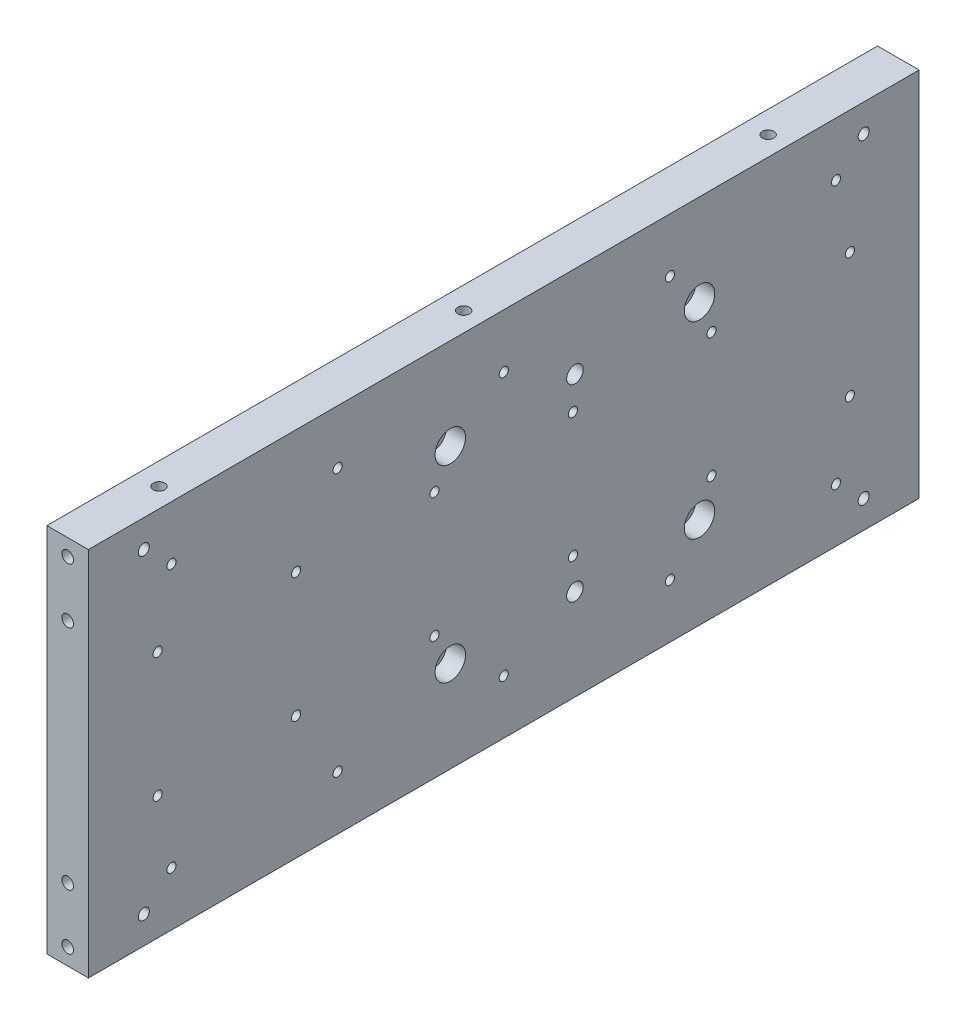
from build123d import *

# Parameters (mm, degrees)
SKETCH1_W                                            = 300
SKETCH1_H                                            = 134
BOSS_EXTRUDE1_DEPTH                                  = 15
M4_TAPPED_HOLE1_D                                    = 3.3
M4_TAPPED_HOLE1_DEPTH                                = 10.1
M4_TAPPED_HOLE1_TIP                                  = 0.991420021
M4_TAPPED_HOLE2_D                                    = 3.3
M4_TAPPED_HOLE2_DEPTH                                = 10.1
M4_TAPPED_HOLE2_TIP                                  = 0.991420021
M5_TAPPED_HOLE1_AT_2_COUNT                           = 2
M5_TAPPED_HOLE1_AT_2_PITCH                           = 20
M5_TAPPED_HOLE1_AT_3_COUNT                           = 2
M5_TAPPED_HOLE1_AT_3_PITCH                           = 102
M5_TAPPED_HOLE1_AT_4_COUNT                           = 2
M5_TAPPED_HOLE1_AT_4_PITCH                           = 122
F_4_0MM_DOWEL_HOLE1_D                                = 4
F_4_0MM_DOWEL_HOLE1_DEPTH                            = 6
F_4_0MM_DOWEL_HOLE1_TIP                              = 1.201721238
CBORE_FOR_M6_HEXAGON_SOCKET_HEAD_CAP_SCR_D           = 6.6
CBORE_FOR_M6_HEXAGON_SOCKET_HEAD_CAP_SCR_CBORE_D     = 11
CBORE_FOR_M6_HEXAGON_SOCKET_HEAD_CAP_SCR_CBORE_DEPTH = 6.8
F_6_0MM_DOWEL_HOLE1_D                                = 6
M5_TAPPED_HOLE2_D                                    = 4.2
M5_TAPPED_HOLE2_DEPTH                                = 12.4
M5_TAPPED_HOLE2_TIP                                  = 1.2618073


with BuildPart() as part:
    # Sketch1 → Boss-Extrude1 (new body)
    with BuildSketch(Plane(origin=(0, 0, 0), x_dir=(0, 0, -1), z_dir=(1, 0, 0))):
        Rectangle(SKETCH1_W, SKETCH1_H)
    extrude(amount=BOSS_EXTRUDE1_DEPTH)

    # M4 Tapped Hole1
    with Locations(Plane(origin=(15, 0, 0), x_dir=(0, 0, -1), z_dir=(1, 0, 0))):
        with Locations((-120, -47.5), (-60, -47.5), (0, -47.5), (60, -47.5), (120, -47.5), (120, 47.5), (60, 47.5), (0, 47.5), (-60, 47.5), (-120, 47.5)):
            Hole(M4_TAPPED_HOLE1_D / 2, depth=M4_TAPPED_HOLE1_DEPTH)
            with Locations((0, 0, -(M4_TAPPED_HOLE1_DEPTH + M4_TAPPED_HOLE1_TIP / 2))):  # 118° drill point
                Cone(0, M4_TAPPED_HOLE1_D / 2, M4_TAPPED_HOLE1_TIP, mode=Mode.SUBTRACT)

    # M4 Tapped Hole2
    with Locations(Plane(origin=(15, 0, 0), x_dir=(0, 0, -1), z_dir=(1, 0, 0))):
        with Locations((-125, 22.5), (-75, 22.5), (-25, 22.5), (-125, -22.5), (-75, -22.5), (-25, -22.5), (25, 22.5), (75, 22.5), (125, 22.5), (125, -22.5), (75, -22.5), (25, -22.5)):
            Hole(M4_TAPPED_HOLE2_D / 2, depth=M4_TAPPED_HOLE2_DEPTH)
            with Locations((0, 0, -(M4_TAPPED_HOLE2_DEPTH + M4_TAPPED_HOLE2_TIP / 2))):  # 118° drill point
                Cone(0, M4_TAPPED_HOLE2_D / 2, M4_TAPPED_HOLE2_TIP, mode=Mode.SUBTRACT)

    # Sketch7 → M5 Tapped Hole1 (revolve, cut)
    with BuildSketch(Plane(origin=(7.5, -61, -150), x_dir=(0, 1, 0), z_dir=(1, 0, 0))):
        Polygon((0, 0), (0, 13.6618073), (2.1, 12.4), (2.1, 0), align=None)
    m5_tapped_hole1 = revolve(axis=Axis((7.5, -61, -156.35), (0, 0, 1)), mode=Mode.SUBTRACT)

    # M5 Tapped Hole1 at 2: M5 Tapped Hole1 ×2
    with Locations(*[(0, i * M5_TAPPED_HOLE1_AT_2_PITCH, 0) for i in range(1, M5_TAPPED_HOLE1_AT_2_COUNT)]):
        add(m5_tapped_hole1, mode=Mode.SUBTRACT)

    # M5 Tapped Hole1 at 3: M5 Tapped Hole1 ×2
    with Locations(*[(0, i * M5_TAPPED_HOLE1_AT_3_PITCH, 0) for i in range(1, M5_TAPPED_HOLE1_AT_3_COUNT)]):
        add(m5_tapped_hole1, mode=Mode.SUBTRACT)

    # M5 Tapped Hole1 at 4: M5 Tapped Hole1 ×2
    with Locations(*[(0, i * M5_TAPPED_HOLE1_AT_4_PITCH, 0) for i in range(1, M5_TAPPED_HOLE1_AT_4_COUNT)]):
        add(m5_tapped_hole1, mode=Mode.SUBTRACT)

    # Mirror1: M5 Tapped Hole1 across plane
    add(m5_tapped_hole1.mirror(Plane.XY), mode=Mode.SUBTRACT)

    # Mirror1 copy 1 sketch → Mirror1 copy 1 (revolve, cut)
    with BuildSketch(Plane(origin=(7.5, -41, 150), x_dir=(0, 1, 0), z_dir=(1, 0, 0))):
        Polygon((0, 0), (0, -13.6618073), (2.1, -12.4), (2.1, 0), align=None)
    revolve(axis=Axis((7.5, -41, 156.35), (0, 0, 1)), mode=Mode.SUBTRACT)

    # Mirror1 copy 2 sketch → Mirror1 copy 2 (revolve, cut)
    with BuildSketch(Plane(origin=(7.5, 41, 150), x_dir=(0, 1, 0), z_dir=(1, 0, 0))):
        Polygon((0, 0), (0, -13.6618073), (2.1, -12.4), (2.1, 0), align=None)
    revolve(axis=Axis((7.5, 41, 156.35), (0, 0, 1)), mode=Mode.SUBTRACT)

    # Mirror1 copy 3 sketch → Mirror1 copy 3 (revolve, cut)
    with BuildSketch(Plane(origin=(7.5, 61, 150), x_dir=(0, 1, 0), z_dir=(1, 0, 0))):
        Polygon((0, 0), (0, -13.6618073), (2.1, -12.4), (2.1, 0), align=None)
    revolve(axis=Axis((7.5, 61, 156.35), (0, 0, 1)), mode=Mode.SUBTRACT)

    # Ø4.0mm Dowel Hole1
    with Locations(Plane(origin=(15, 0, 0), x_dir=(0, 0, -1), z_dir=(1, 0, 0))):
        with Locations((130, 57), (-130, 57), (-130, -57), (130, -57)):
            Hole(F_4_0MM_DOWEL_HOLE1_D / 2, depth=F_4_0MM_DOWEL_HOLE1_DEPTH)
            with Locations((0, 0, -(F_4_0MM_DOWEL_HOLE1_DEPTH + F_4_0MM_DOWEL_HOLE1_TIP / 2))):  # 118° drill point
                Cone(0, F_4_0MM_DOWEL_HOLE1_D / 2, F_4_0MM_DOWEL_HOLE1_TIP, mode=Mode.SUBTRACT)

    # CBORE for M6 Hexagon socket head cap screws1 (through all)
    with Locations(Plane(origin=(15, 0, 0), x_dir=(0, 0, -1), z_dir=(1, 0, 0))):
        with Locations((70.7, 34), (-19.3, 34), (-19.3, -34), (70.7, -34)):
            CounterBoreHole(CBORE_FOR_M6_HEXAGON_SOCKET_HEAD_CAP_SCR_D / 2, CBORE_FOR_M6_HEXAGON_SOCKET_HEAD_CAP_SCR_CBORE_D / 2, CBORE_FOR_M6_HEXAGON_SOCKET_HEAD_CAP_SCR_CBORE_DEPTH)

    # Ø6.0mm Dowel Hole1 (through all)
    with Locations(Plane(origin=(15, 0, 0), x_dir=(0, 0, -1), z_dir=(1, 0, 0))):
        with Locations((25.7, 34), (25.7, -34)):
            Hole(F_6_0MM_DOWEL_HOLE1_D / 2)

    # M5 Tapped Hole2
    with Locations(Plane(origin=(0, 67, 0), x_dir=(-1, 0, 0), z_dir=(0, 1, 0))):
        with Locations((-8, 117.5), (-8, -102.5), (-8, 7.5)):
            Hole(M5_TAPPED_HOLE2_D / 2, depth=M5_TAPPED_HOLE2_DEPTH)
            with Locations((0, 0, -(M5_TAPPED_HOLE2_DEPTH + M5_TAPPED_HOLE2_TIP / 2))):  # 118° drill point
                Cone(0, M5_TAPPED_HOLE2_D / 2, M5_TAPPED_HOLE2_TIP, mode=Mode.SUBTRACT)


solid = part.part
